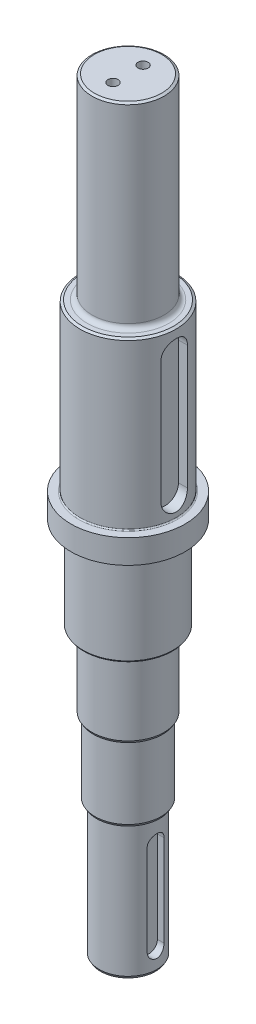
from build123d import *
from OCP.BRepFilletAPI import BRepFilletAPI_MakeChamfer

# Parameters (mm, degrees)
CHAMFER1_SIZE          = 2
CHAMFER1_SIZE2         = 1.154700538
FILLET1_R              = 1
FILLET2_R              = 4
FILLET3_R              = 5
CHAMFER2_SIZE          = 1
CHAMFER2_SIZE2         = 0.577350269
CHAMFER3_SIZE          = 2
CHAMFER3_SIZE2         = 1.154700538
CHAMFER4_SIZE          = 2
CHAMFER4_SIZE2         = 1.154700538
M10_TAPPED_HOLE1_D     = 8.5
M10_TAPPED_HOLE1_DEPTH = 24.5
M10_TAPPED_HOLE1_TIP   = 2.553657631
CUT_EXTRUDE1_START     = 94
CUT_EXTRUDE1_DEPTH     = 63
CUT_EXTRUDE2_START     = 17.46
CUT_EXTRUDE2_DEPTH     = 63


with BuildPart() as part:
    # Sketch2 → Revolve1 (revolve)
    with BuildSketch(Plane.XY, mode=Mode.PRIVATE) as revolve1_sk:
        Polygon((0, -318), (0, 318), (30, 318), (30, 155), (40, 155), (40, 17), (47.5, 17), (47.5, -3), (37.5, -3), (37.5, -80), (30, -80), (30, -144), (27.5, -144), (27.5, -206), (24, -206), (24, -318), align=None)
    revolve(revolve1_sk.sketch.rotate(Axis((0, -318, 0), (0, 1, 0)), 90), axis=Axis((0, -318, 0), (0, 1, 0)))

    # Chamfer1: one chamfer whose edges measure the first distance from different faces: ONE call of the kernel's chamfer builder (chamfer() names one face for all edges)
    chamfer1_edges_1 = [part.edges().sort_by_distance(p)[0] for p in [
        (0, -318, 24),
    ]]
    chamfer1_side_1 = [part.faces().sort_by_distance(p)[0] for p in [
        (0, -262, 24),
    ]]
    chamfer1_edges_2 = [part.edges().sort_by_distance(p)[0] for p in [
        (0, 155, 40),
    ]]
    chamfer1_side_2 = [part.faces().sort_by_distance(p)[0] for p in [
        (0, 155, 31.13137085),
    ]]
    chamfer1_edges_3 = [part.edges().sort_by_distance(p)[0] for p in [
        (0, 318, 30),
    ]]
    chamfer1_side_3 = [part.faces().sort_by_distance(p)[0] for p in [
        (0, 318, 0),
    ]]
    chamfer1 = BRepFilletAPI_MakeChamfer(part.part.solid().wrapped)
    for e in chamfer1_edges_1:
        chamfer1.Add(CHAMFER1_SIZE, CHAMFER1_SIZE2, e.wrapped, chamfer1_side_1[0].wrapped)  # the first distance lies on this face
    for e in chamfer1_edges_2:
        chamfer1.Add(CHAMFER1_SIZE, CHAMFER1_SIZE2, e.wrapped, chamfer1_side_2[0].wrapped)  # the first distance lies on this face
    for e in chamfer1_edges_3:
        chamfer1.Add(CHAMFER1_SIZE, CHAMFER1_SIZE2, e.wrapped, chamfer1_side_3[0].wrapped)  # the first distance lies on this face
    add(Compound.cast(chamfer1.Shape()), mode=Mode.REPLACE)

    # Fillet1
    fillet1_edges = [part.edges().sort_by_distance(p)[0] for p in [
        (0, -206, 24),
        (0, -144, 27.5),
        (0, -80, 30),
        (0, 17, 40),
    ]]
    fillet(fillet1_edges, radius=FILLET1_R)

    # Fillet2
    fillet2_edges = [part.edges().sort_by_distance(p)[0] for p in [
        (0, 155, 30),
    ]]
    fillet(fillet2_edges, radius=FILLET2_R)

    # Fillet3
    fillet3_edges = [part.edges().sort_by_distance(p)[0] for p in [
        (0, -3, 37.5),
    ]]
    fillet(fillet3_edges, radius=FILLET3_R)

    # Chamfer2
    chamfer2_edges = [part.edges().sort_by_distance(p)[0] for p in [
        (0, -80, 37.5),
    ]]
    chamfer2_side = [part.faces().sort_by_distance(p)[0] for p in [
        (0, -44, 37.5),
    ]]
    chamfer(chamfer2_edges, length=CHAMFER2_SIZE, length2=CHAMFER2_SIZE2, reference=chamfer2_side[0])

    # Chamfer3
    chamfer3_edges = [part.edges().sort_by_distance(p)[0] for p in [
        (0, -206, 27.5),
    ]]
    chamfer3_side = [part.faces().sort_by_distance(p)[0] for p in [
        (0, -175.5, 27.5),
    ]]
    chamfer(chamfer3_edges, length=CHAMFER3_SIZE, length2=CHAMFER3_SIZE2, reference=chamfer3_side[0])

    # Chamfer4
    chamfer4_edges = [part.edges().sort_by_distance(p)[0] for p in [
        (0, -144, 30),
    ]]
    chamfer4_side = [part.faces().sort_by_distance(p)[0] for p in [
        (0, -112.5, 30),
    ]]
    chamfer(chamfer4_edges, length=CHAMFER4_SIZE, length2=CHAMFER4_SIZE2, reference=chamfer4_side[0])

    # M10 Tapped Hole1
    with Locations(Plane(origin=(0, 318, 0), x_dir=(1, 0, 0), z_dir=(0, 1, 0))):
        with Locations((0, 12.5), (0, -12.5)):
            Hole(M10_TAPPED_HOLE1_D / 2, depth=M10_TAPPED_HOLE1_DEPTH)
            with Locations((0, 0, -(M10_TAPPED_HOLE1_DEPTH + M10_TAPPED_HOLE1_TIP / 2))):  # 118° drill point
                Cone(0, M10_TAPPED_HOLE1_D / 2, M10_TAPPED_HOLE1_TIP, mode=Mode.SUBTRACT)

    # Sketch6 → Cut-Extrude1 (cut)
    with BuildSketch(Plane(origin=(0, 0, 0), x_dir=(0, 0, -1), z_dir=(1, 0, 0)).offset(CUT_EXTRUDE1_START)):
        with BuildLine():
            Line((11, 136), (11, 33))
            ThreePointArc((11, 33), (0, 22), (-11, 33))
            Line((-11, 33), (-11, 136))
            ThreePointArc((-11, 136), (0, 147), (11, 136))
        make_face()
    extrude(amount=-CUT_EXTRUDE1_DEPTH, mode=Mode.SUBTRACT)

    # Sketch8 → Cut-Extrude2 (cut)
    with BuildSketch(Plane(origin=(0, 0, 0), x_dir=(0, 0, -1), z_dir=(1, 0, 0)).offset(CUT_EXTRUDE2_START)):
        with BuildLine():
            Line((-7, -301), (-7, -225))
            ThreePointArc((-7, -225), (0, -218), (7, -225))
            Line((7, -225), (7, -301))
            ThreePointArc((7, -301), (0, -308), (-7, -301))
        make_face()
    extrude(amount=CUT_EXTRUDE2_DEPTH, mode=Mode.SUBTRACT)


solid = part.part
